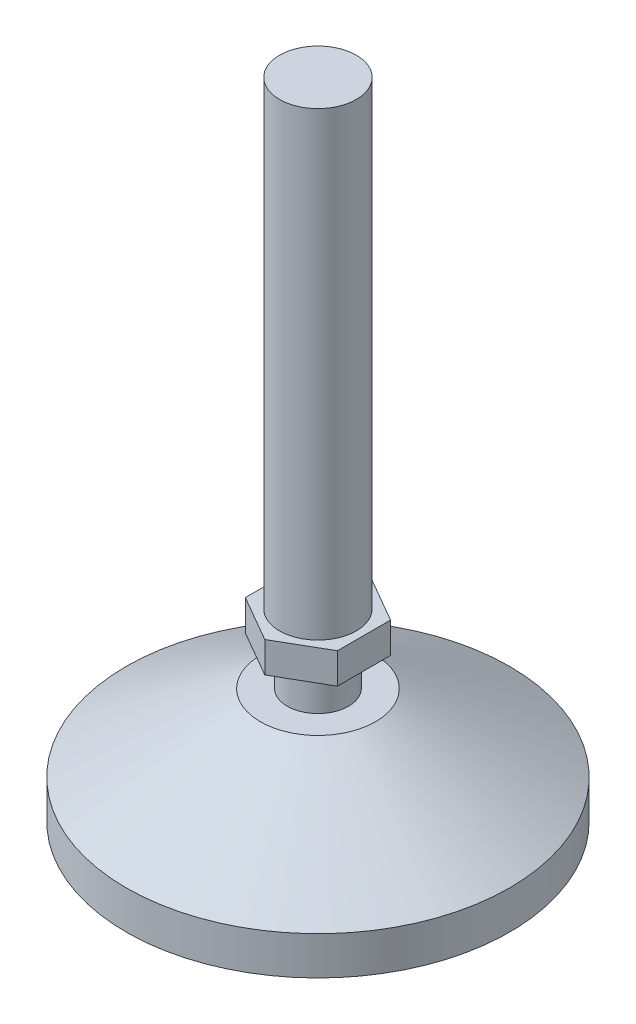
SolidWorks part; units mm, degrees
ref_plane "前视基准面" through (0, 0, 0) normal (0, 0, 1) x (1, 0, 0)
ref_plane "上视基准面" through (0, 0, 0) normal (0, 1, 0) x (1, 0, 0)
ref_plane "右视基准面" through (0, 0, 0) normal (1, 0, 0) x (0, 0, -1)
sketch "草图1" plane through (0, 0, 0) normal (0, 0, 1) x (1, 0, 0)
  line L0 (0, 30) -> (0, 0)
  line L1 (0, 0) -> (50, 0)
  line L2 (50, 0) -> (50, 10)
  line L3 (50, 10) -> (15, 30)
  line L4 (15, 30) -> (0, 30)
  dimension "D1" = 15
  dimension "D2" = 30
  dimension "D3" = 50
  dimension "D4" = 10
revolve "旋转1" add sketch "草图1" angle 360 about L0
sketch "草图2" plane through (0, 30, 0) normal (0, 1, 0) x (1, 0, 0)
  circle A0 centre (0, 0) radius 8
  dimension "D1" = 16
extrude "凸台-拉伸1" add sketch "草图2" along normal blind 10
sketch "草图3" plane through (0, 40, 0) normal (0, 1, 0) x (1, 0, 0)
  line L0 (0, 0) -> (0, 23.0176) construction
  line L1 (0, 13.8564) -> (-12, 6.9282)
  line L2 (-12, 6.9282) -> (-12, -6.9282)
  line L3 (-12, -6.9282) -> (0, -13.8564)
  line L4 (0, -13.8564) -> (12, -6.9282)
  line L5 (12, -6.9282) -> (12, 6.9282)
  line L6 (12, 6.9282) -> (0, 13.8564)
  circle A0 centre (0, 0) radius 12 construction
  dimension "D1" = 24
extrude "凸台-拉伸2" add sketch "草图3" along normal blind 8
sketch "草图4" plane through (0, 48, 0) normal (0, 1, 0) x (1, 0, 0)
  circle A0 centre (0, 0) radius 10
  dimension "D1" = 20
extrude "凸台-拉伸3" add sketch "草图4" along normal blind 120
